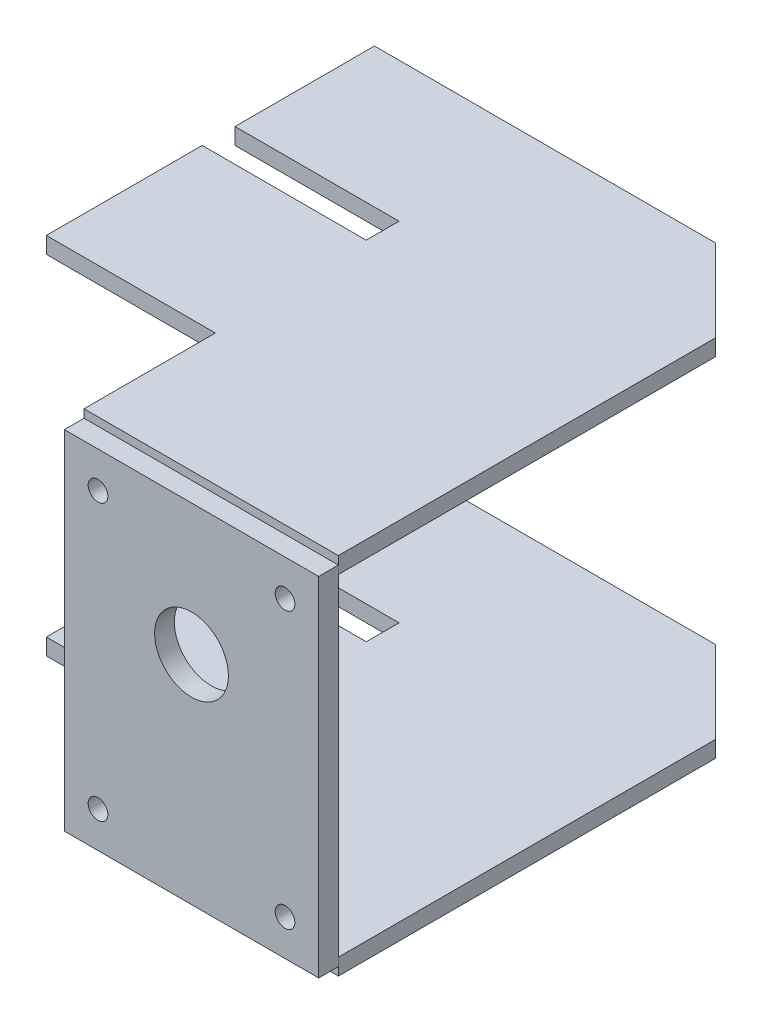
from build123d import *

# Parameters (mm, degrees)
SKETCH1_W           = 155
SKETCH1_H           = 212
BOSS_EXTRUDE1_DEPTH = 12
F_12_0_12_HOLE1_D   = 12
BOSS_EXTRUDE2_DEPTH = 5
CHAMFER1_SIZE       = 50
SKETCH9_R           = 22.5
CUT_EXTRUDE1_DEPTH  = 12
SKETCH10_W          = 100
SKETCH10_H          = 20
CUT_EXTRUDE2_DEPTH  = 401.33017623


with BuildPart() as part:
    # Sketch1 → Boss-Extrude1 (new body)
    with BuildSketch(Plane.XY):
        Rectangle(SKETCH1_W, SKETCH1_H)
    extrude(amount=BOSS_EXTRUDE1_DEPTH)

    # Ø12.0 (12) Hole1 (through all)
    with Locations(Plane(origin=(0, 0, 0), x_dir=(-1, 0, 0), z_dir=(0, 0, -1))):
        with Locations((-57, 84), (57, 84), (-57, -84), (57, -84)):
            Hole(F_12_0_12_HOLE1_D / 2)

    # Sketch9 → Cut-Extrude1 (cut)
    with BuildSketch(Plane(origin=(0, 0, 0), x_dir=(-1, 0, 0), z_dir=(0, 0, -1))):
        with Locations((0, 26)):
            Circle(SKETCH9_R)
    extrude(amount=-CUT_EXTRUDE1_DEPTH, mode=Mode.SUBTRACT)


with BuildPart() as body_2:
    # Sketch8 → Boss-Extrude2 (new, symmetric)
    with BuildSketch(Plane(origin=(0, 106, 0), x_dir=(1, 0, 0), z_dir=(0, 1, 0))):
        Polygon((77.5, 0), (-77.5, 0), (-77.5, 80), (-180.5, 80), (-180.5, 280), (77.5, 280), align=None)
    extrude(amount=BOSS_EXTRUDE2_DEPTH, both=True)

    # Chamfer1
    chamfer1_edges = [body_2.edges().sort_by_distance(p)[0] for p in [
        (77.5, 106, -280),
    ]]
    chamfer(chamfer1_edges, length=CHAMFER1_SIZE)


with BuildPart() as body_3:
    # Mirror1: mirrored copy
    add(body_2.part.mirror(Plane.ZX))


with BuildPart() as cut_extrude2_tool:
    # Sketch10 → Cut-Extrude2 (new, through all)
    with BuildSketch(Plane(origin=(0, 111, 0), x_dir=(1, 0, 0), z_dir=(0, 1, 0))):
        with Locations((-130.5, 185)):
            Rectangle(SKETCH10_W, SKETCH10_H)
    extrude(amount=-CUT_EXTRUDE2_DEPTH)


with BuildPart() as body_2_1:
    add(body_2.part)

    # Cut-Extrude2: cut by cut_extrude2_tool
    add(cut_extrude2_tool.part, mode=Mode.SUBTRACT)


with BuildPart() as body_3_1:
    add(body_3.part)

    # Cut-Extrude2: cut by cut_extrude2_tool
    add(cut_extrude2_tool.part, mode=Mode.SUBTRACT)


solid = Compound([part.part, body_2_1.part, body_3_1.part])
